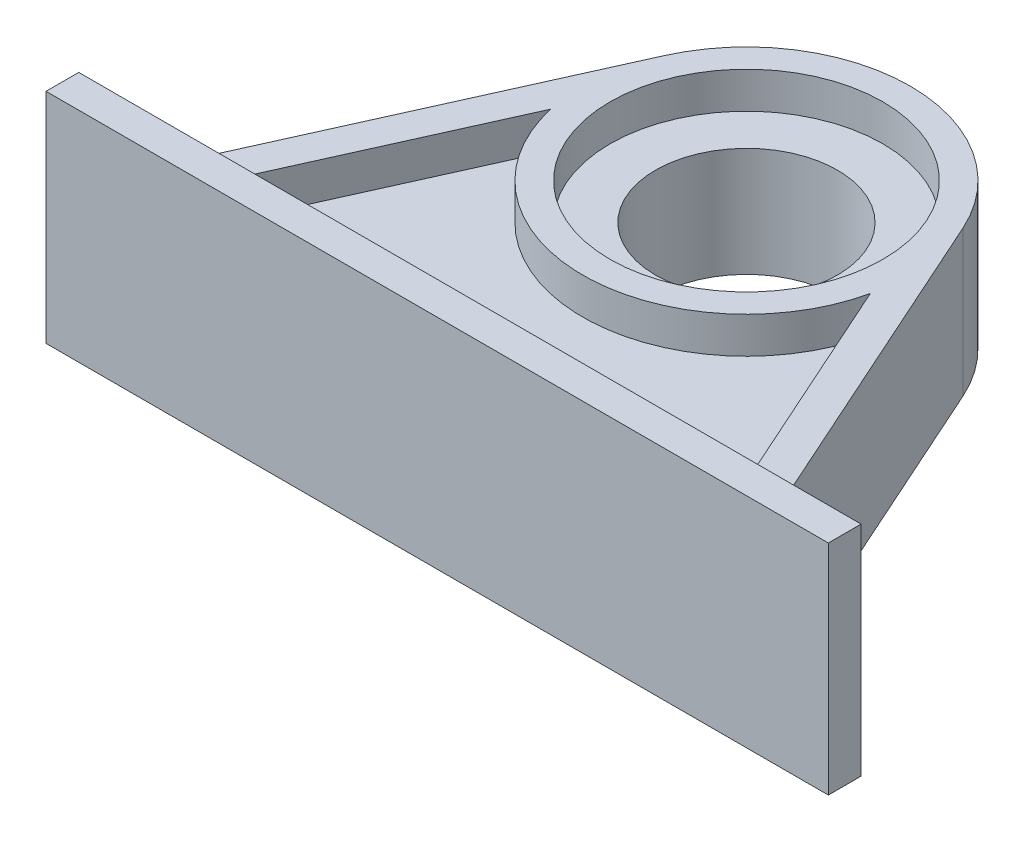
from build123d import *

# Parameters (mm, degrees)
BOSS_EXTRUDE1_DEPTH      = 40
BOSS_EXTRUDE1_DEPTH_BACK = 40
SKETCH1_R                = 50
CUT_EXTRUDE1_START       = -20
SKETCH2_R                = 75
SKETCH2_R_2              = 50
CUT_EXTRUDE1_DEPTH       = 20
CUT_EXTRUDE2_START       = -20
CUT_EXTRUDE2_DEPTH       = 20
BOSS_EXTRUDE2_DEPTH      = 20
BOSS_EXTRUDE2_DEPTH_BACK = 100
SKETCH4_W                = 430
SKETCH4_H                = 18
SKETCH5_R                = 15
BOSS_EXTRUDE3_DEPTH      = 4
BOSS_EXTRUDE4_DEPTH      = 10


with BuildPart() as part:
    # Sketch1 → Boss-Extrude1 (new, two sides: drawn at the far end of the back side and taken through both)
    with BuildSketch(Plane(origin=(0, 0, 0), x_dir=(1, 0, 0), z_dir=(0, 1, 0)).offset(-BOSS_EXTRUDE1_DEPTH_BACK)):
        with BuildLine():
            Line((-175, -170), (175, -170))
            Line((175, -170), (82.10152682, 36.869218785))
            ThreePointArc((82.10152682, 36.869218785), (0, 90), (-82.10152682, 36.869218785))
            Line((-82.10152682, 36.869218785), (-175, -170))
        make_face()
        with Locations(Location((0, 0, 0), (0, 0, 270))):
            Circle(SKETCH1_R, mode=Mode.SUBTRACT)
    extrude(amount=BOSS_EXTRUDE1_DEPTH + BOSS_EXTRUDE1_DEPTH_BACK)

    # Sketch2 → Cut-Extrude1 (cut)
    with BuildSketch(Plane(origin=(0, 40, 0), x_dir=(1, 0, 0), z_dir=(0, 1, 0)).offset(CUT_EXTRUDE1_START)):
        with Locations(Location((0, 0, 0), (0, 0, 270))):
            Circle(SKETCH2_R)
        with Locations(Location((0, 0, 0), (0, 0, 270))):
            Circle(SKETCH2_R_2, mode=Mode.SUBTRACT)
    extrude(amount=CUT_EXTRUDE1_DEPTH, mode=Mode.SUBTRACT)

    # Sketch3 → Cut-Extrude2 (cut)
    with BuildSketch(Plane(origin=(0, 40, 0), x_dir=(1, 0, 0), z_dir=(0, 1, 0)).offset(CUT_EXTRUDE2_START)):
        with BuildLine():
            Line((-87.802752727, -19.765541064), (-147.18509781, -152))
            Line((-147.18509781, -152), (147.18509781, -152))
            Line((147.18509781, -152), (87.802752727, -19.765541064))
            ThreePointArc((87.802752727, -19.765541064), (0, -90), (-87.802752727, -19.765541064))
        make_face()
    cut_extrude2 = extrude(amount=CUT_EXTRUDE2_DEPTH, mode=Mode.SUBTRACT)

    # Mirror1: Cut-Extrude2 across plane
    add(cut_extrude2.mirror(Plane.ZX), mode=Mode.SUBTRACT)

    # Sketch4 → Boss-Extrude2 (add, two sides: drawn at the far end of the back side and taken through both)
    with BuildSketch(Plane(origin=(0, 40, 0), x_dir=(1, 0, 0), z_dir=(0, 1, 0)).offset(-BOSS_EXTRUDE2_DEPTH_BACK)):
        with Locations((0, -161)):
            Rectangle(SKETCH4_W, SKETCH4_H)
    extrude(amount=BOSS_EXTRUDE2_DEPTH + BOSS_EXTRUDE2_DEPTH_BACK)

    # Sketch5 → Boss-Extrude3 (add)
    with BuildSketch(Plane(origin=(0, 0, 152), x_dir=(-1, 0, 0), z_dir=(0, 0, -1))):
        with Locations(Location((-190, 35, 0), (0, 0, 180))):
            Circle(SKETCH5_R)
        with Locations(Location((-190, -35, 0), (0, 0, 180))):
            Circle(SKETCH5_R)
        with Locations(Location((190, -35, 0), (0, 0, 180))):
            Circle(SKETCH5_R)
        with Locations(Location((190, 35, 0), (0, 0, 180))):
            Circle(SKETCH5_R)
    extrude(amount=BOSS_EXTRUDE3_DEPTH)

    # Sketch6 → Boss-Extrude4 (add)
    with BuildSketch(Plane(origin=(0, 0, 148), x_dir=(-1, 0, 0), z_dir=(0, 0, -1))):
        Polygon((-179.344928978, 35), (-184.672464489, 44.227562184), (-195.327535511, 44.227562184), (-200.655071022, 35), (-195.327535511, 25.772437816), (-184.672464489, 25.772437816), align=None)
        Polygon((-179.344928978, -38.24088904), (-181.86577225, -27.392882336), (-192.520843272, -24.151993296), (-200.655071022, -31.75911096), (-198.13422775, -42.607117664), (-187.479156728, -45.848006704), align=None)
        Polygon((199.191466328, 30.386218908), (198.591384797, 40.653152792), (189.399918469, 45.266933884), (180.808533672, 39.613781092), (181.408615203, 29.346847208), (190.600081531, 24.733066116), align=None)
        Polygon((199.191466328, -38.24088904), (197.402425403, -28.660401182), (188.210959075, -25.419512142), (180.808533672, -31.75911096), (182.597574597, -41.339598818), (191.789040925, -44.580487858), align=None)
    extrude(amount=BOSS_EXTRUDE4_DEPTH)


solid = part.part
